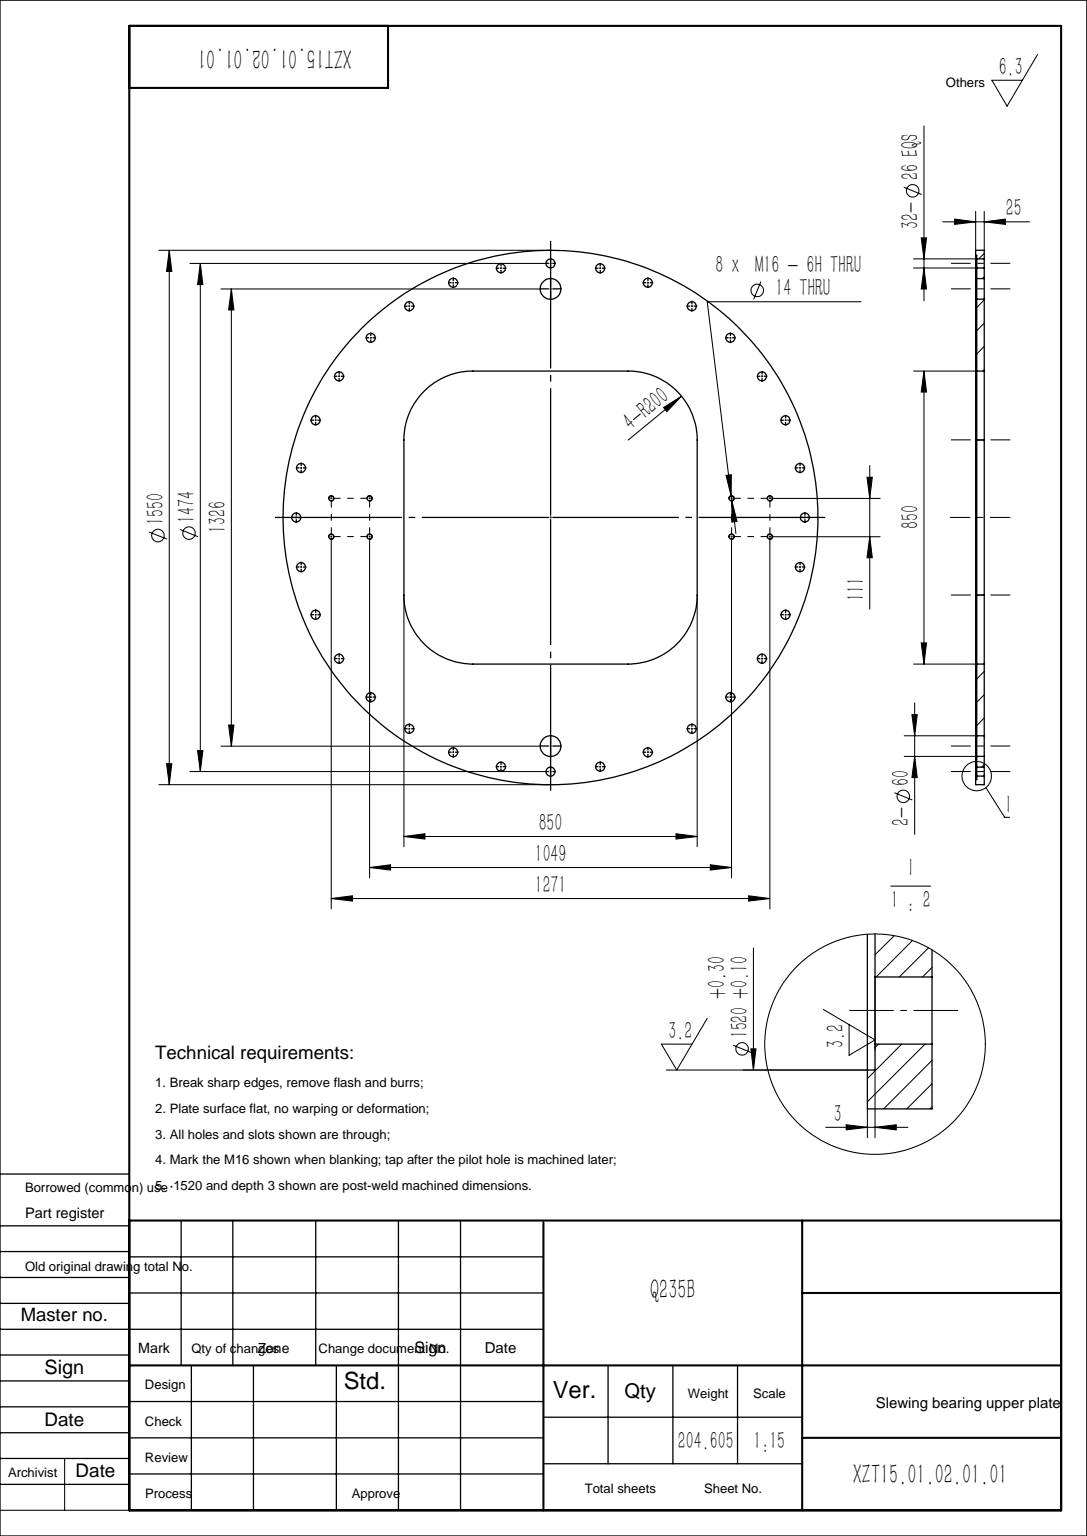
SolidWorks part; units mm, degrees
material "Q235B"
ref_plane "Front Plane" through (0, 0, 0) normal (0, 0, 1) x (1, 0, 0)
ref_plane "Top Plane" through (0, 0, 0) normal (0, 1, 0) x (1, 0, 0)
ref_plane "Right Plane" through (0, 0, 0) normal (1, 0, 0) x (0, 0, -1)
sketch "Sketch1" plane through (0, 0, 0) normal (0, 1, 0) x (1, 0, 0)
  line L0 (0, 0) -> (0, 663) construction
  line L1 (225, -425) -> (-225, -425)
  line L2 (425, -225) -> (425, 225)
  line L3 (225, 425) -> (-225, 425)
  line L4 (-425, -225) -> (-425, 225)
  line L5 (425, -425) -> (-425, 425) construction
  line L6 (425, 425) -> (-425, -425) construction
  line L7 (0, 0) -> (-1232.836, 0) construction
  line L8 (0, 0) -> (0, 737) construction
  circle A0 centre (0, 0) radius 775
  arc A1 (-225, -425) -> (-425, -225) centre (-225, -225) cw
  arc A2 (425, 225) -> (225, 425) centre (225, 225) ccw
  arc A3 (225, -425) -> (425, -225) centre (225, -225) ccw
  arc A4 (-225, 425) -> (-425, 225) centre (-225, 225) ccw
  circle A5 centre (0, 663) radius 30
  circle A6 centre (0, -663) radius 30
  circle A7 centre (0, 737) radius 13
  circle A8 centre (143.7816, 722.8388) radius 13
  circle A9 centre (282.0377, 680.8992) radius 13
  circle A10 centre (409.4553, 612.7931) radius 13
  circle A11 centre (521.1377, 521.1377) radius 13
  circle A12 centre (612.7931, 409.4553) radius 13
  circle A13 centre (680.8992, 282.0377) radius 13
  circle A14 centre (722.8388, 143.7816) radius 13
  circle A15 centre (737, 0) radius 13
  circle A16 centre (722.8388, -143.7816) radius 13
  circle A17 centre (680.8992, -282.0377) radius 13
  circle A18 centre (612.7931, -409.4553) radius 13
  circle A19 centre (521.1377, -521.1377) radius 13
  circle A20 centre (409.4553, -612.7931) radius 13
  circle A21 centre (282.0377, -680.8992) radius 13
  circle A22 centre (143.7816, -722.8388) radius 13
  circle A23 centre (0, -737) radius 13
  circle A24 centre (-143.7816, -722.8388) radius 13
  circle A25 centre (-282.0377, -680.8992) radius 13
  circle A26 centre (-409.4553, -612.7931) radius 13
  circle A27 centre (-521.1377, -521.1377) radius 13
  circle A28 centre (-612.7931, -409.4553) radius 13
  circle A29 centre (-680.8992, -282.0377) radius 13
  circle A30 centre (-722.8388, -143.7816) radius 13
  circle A31 centre (-737, 0) radius 13
  circle A32 centre (-722.8388, 143.7816) radius 13
  circle A33 centre (-680.8992, 282.0377) radius 13
  circle A34 centre (-612.7931, 409.4553) radius 13
  circle A35 centre (-521.1377, 521.1377) radius 13
  circle A36 centre (-409.4553, 612.7931) radius 13
  circle A37 centre (-282.0377, 680.8992) radius 13
  circle A38 centre (-143.7816, 722.8388) radius 13
  point P91 (0, 0)
  dimension "D1" = 1550
  dimension "D3" = 200
  dimension "D4" = 60
  dimension "D5" = 1326
  dimension "D6" = 26
  dimension "D2" = 850
  dimension "D7" = 1474
  dimension "D8" = 32
extrude "Boss-Extrude1" add sketch "Sketch1" along normal blind 25
hole_wizard "M16 Tapped Hole1" positions "Sketch2" profile "Sketch3" tap size "M16" standard "GB" end condition up to next
sketch "Sketch2" plane through (0, 25, 0) normal (0, 1, 0) x (1, 0, 0)
  line L0 (0, 0) -> (0, 775) construction
  line L1 (0, 0) -> (-737, 0) construction
  circle A0 centre (0, 0) radius 775 construction
  point P0 (-635.5, -55.5)
  point P12 (-524.5, -55.5)
  point P13 (-524.5, 55.5)
  point P14 (-635.5, 55.5)
  point P17 (635.5, 55.5)
  point P18 (524.5, 55.5)
  point P19 (524.5, -55.5)
  point P20 (635.5, -55.5)
  dimension "D1" = 2
  dimension "D3" = 1049
  dimension "D4" = 1271
  dimension "D5" = 111
  dimension "D2" = 2
sketch "Sketch3" plane through (-635.5, 25, 55.5) normal (1, 0, 0) x (0, 0, 1)
  line L0 (0, 0) -> (0, 25)
  line L1 (0, 25) -> (7, 25)
  line L2 (7, 25) -> (7, 0)
  line L5 (7, 0) -> (0, 0)
  line L11 (0, -6.35) -> (0, 107.95) construction
  dimension "通孔螺纹孔钻头直径" = 14
  dimension "通孔螺纹孔钻头深度" = 25
cosmetic thread "Cosmetic Thread 1" parameters "D2"=16
cosmetic thread "Cosmetic Thread 2" parameters "D2"=16
cosmetic thread "Cosmetic Thread 3" parameters "D2"=16
cosmetic thread "Cosmetic Thread 4" parameters "D2"=16
cosmetic thread "Cosmetic Thread 5" parameters "D2"=16
cosmetic thread "Cosmetic Thread 6" parameters "D2"=16
cosmetic thread "Cosmetic Thread 7" parameters "D2"=16
cosmetic thread "Cosmetic Thread 8" parameters "D2"=16
sketch "Sketch4" plane through (0, 0, 0) normal (0, -1, 0) x (1, 0, 0)
  circle A0 centre (0, 0) radius 760
  dimension "D1" = 1520
extrude "Cut-Extrude1" cut sketch "Sketch4" against normal blind 3
